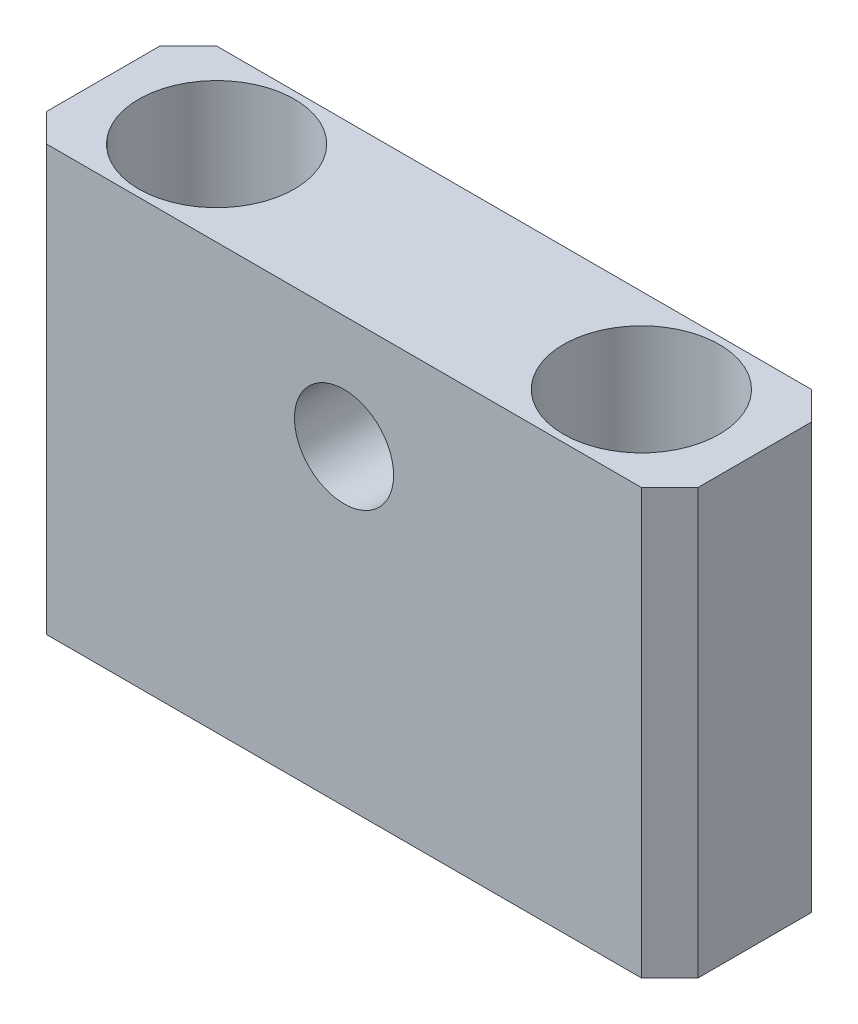
from build123d import *

# Parameters (mm, degrees)
SKETCH_1_W                   = 46
SKETCH_1_H                   = 30
EXTRUDE_1_DEPTH              = 12
HOLE_WIZARD_7_0_7_1_D        = 7
HOLE_WIZARD_M6_1_D           = 6.4
HOLE_WIZARD_M6_1_CBORE_D     = 11
HOLE_WIZARD_M6_1_CBORE_DEPTH = 6.4
SKETCH_7_R                   = 5.5
CUT_EXTRUDE_1_DEPTH          = 10
CHAMFER_1_SIZE               = 2


with BuildPart() as part:
    # 草图1 → 凸台-拉伸1 (new body)
    with BuildSketch(Plane.XY):
        with Locations((23, 15)):
            Rectangle(SKETCH_1_W, SKETCH_1_H)
    extrude(amount=EXTRUDE_1_DEPTH)

    # Ø7.0 (7) 直径孔1 (through all)
    with Locations(Plane.XY.offset(12)):
        with Locations((23, 22)):
            Hole(HOLE_WIZARD_7_0_7_1_D / 2)

    # M6 六角凹头螺钉的柱形沉头孔1 (through all)
    with Locations(Plane(origin=(0, 30, 0), x_dir=(1, 0, 0), z_dir=(0, 1, 0))):
        with Locations((8, -6), (38, -6)):
            CounterBoreHole(HOLE_WIZARD_M6_1_D / 2, HOLE_WIZARD_M6_1_CBORE_D / 2, HOLE_WIZARD_M6_1_CBORE_DEPTH)

    # 草图7 → 切除-拉伸1 (cut)
    with BuildSketch(Plane(origin=(0, 23.6, 0), x_dir=(1, 0, 0), z_dir=(0, 1, 0))):
        with Locations(Location((8, -6, 0), (0, 0, 270))):
            Circle(SKETCH_7_R)
        with Locations(Location((38, -6, 0), (0, 0, 270))):
            Circle(SKETCH_7_R)
    extrude(amount=-CUT_EXTRUDE_1_DEPTH, mode=Mode.SUBTRACT)

    # 倒角1
    chamfer_1_edges = [part.edges().sort_by_distance(p)[0] for p in [
        (46, 15, 12),
        (0, 15, 12),
        (46, 15, 0),
        (0, 15, 0),
    ]]
    chamfer(chamfer_1_edges, length=CHAMFER_1_SIZE)


solid = part.part
